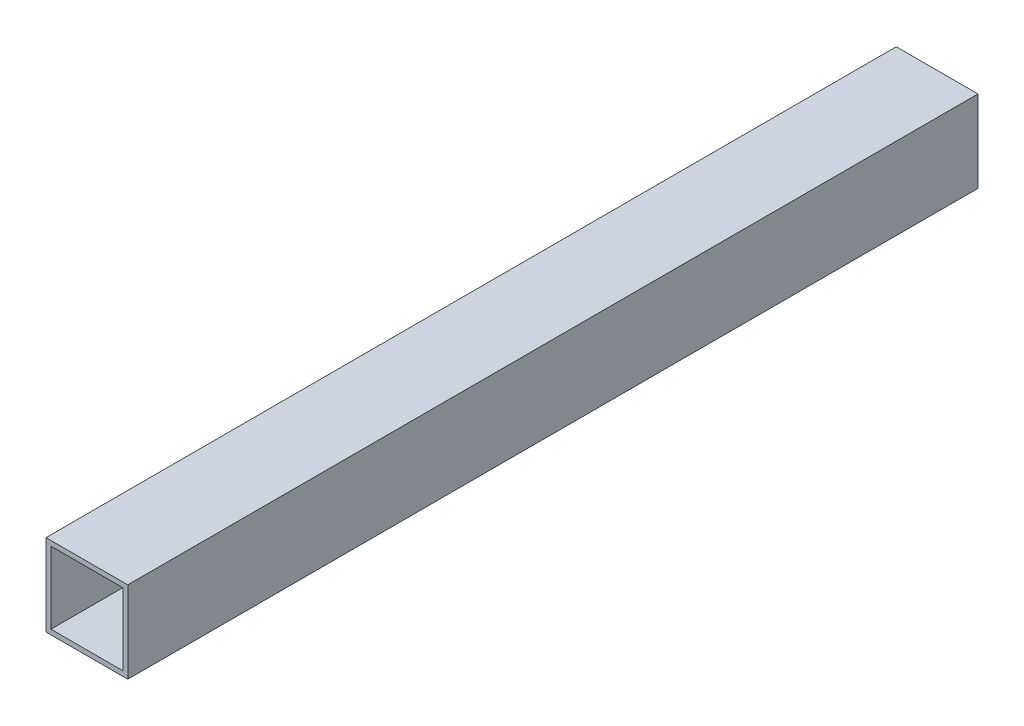
SolidWorks part; units mm, degrees
ref_plane "前视基准面" through (0, 0, 0) normal (0, 0, 1) x (1, 0, 0)
ref_plane "上视基准面" through (0, 0, 0) normal (0, 1, 0) x (1, 0, 0)
ref_plane "右视基准面" through (0, 0, 0) normal (1, 0, 0) x (0, 0, -1)
sketch "草图1" plane through (0, 0, 0) normal (0, 0, 1) x (1, 0, 0)
  line L0 (0, 0) -> (0, 50)
  line L1 (0, 50) -> (50, 50)
  line L2 (50, 50) -> (50, 0)
  line L3 (50, 0) -> (0, 0)
  line L4 (3, 3) -> (3, 47)
  line L5 (3, 47) -> (47, 47)
  line L6 (47, 47) -> (47, 3)
  line L7 (47, 3) -> (3, 3)
  dimension "D1" = 3
extrude "凸台-拉伸1" add sketch "草图1" along normal blind 520
sketch "草图2" plane through (0, 0, 520) normal (0, 0, 1) x (1, 0, 0)
  line L8 (-3, -3) -> (53, -3)
  line L9 (53, -3) -> (53, 53)
  line L10 (53, 53) -> (-3, 53)
  line L11 (-3, 53) -> (-3, -3)
  line L12 (-3, -3) -> (53, -3)
  line L13 (53, -3) -> (53, 53)
  line L14 (53, 53) -> (-3, 53)
  line L15 (-3, 53) -> (-3, -3)
  dimension "D1" = 3
extrude "切除-拉伸1" cut sketch "草图2" against normal blind 100
sketch "草图3" plane through (0, 0, 420) normal (0, 0, 1) x (1, 0, 0)
  line L4 (3, 47) -> (47, 47)
  line L5 (47, 47) -> (47, 3)
  line L6 (47, 3) -> (3, 3)
  line L7 (3, 3) -> (3, 47)
  line L8 (0, 0) -> (50, 0)
  line L9 (50, 0) -> (50, 50)
  line L10 (50, 50) -> (0, 50)
  line L11 (0, 50) -> (0, 0)
  line L12 (0, 0) -> (50, 0)
  line L13 (50, 0) -> (50, 50)
  line L14 (50, 50) -> (0, 50)
  line L15 (0, 50) -> (0, 0)
  dimension "D1" = 0
extrude "凸台-拉伸2" add sketch "草图3" along normal blind 100
